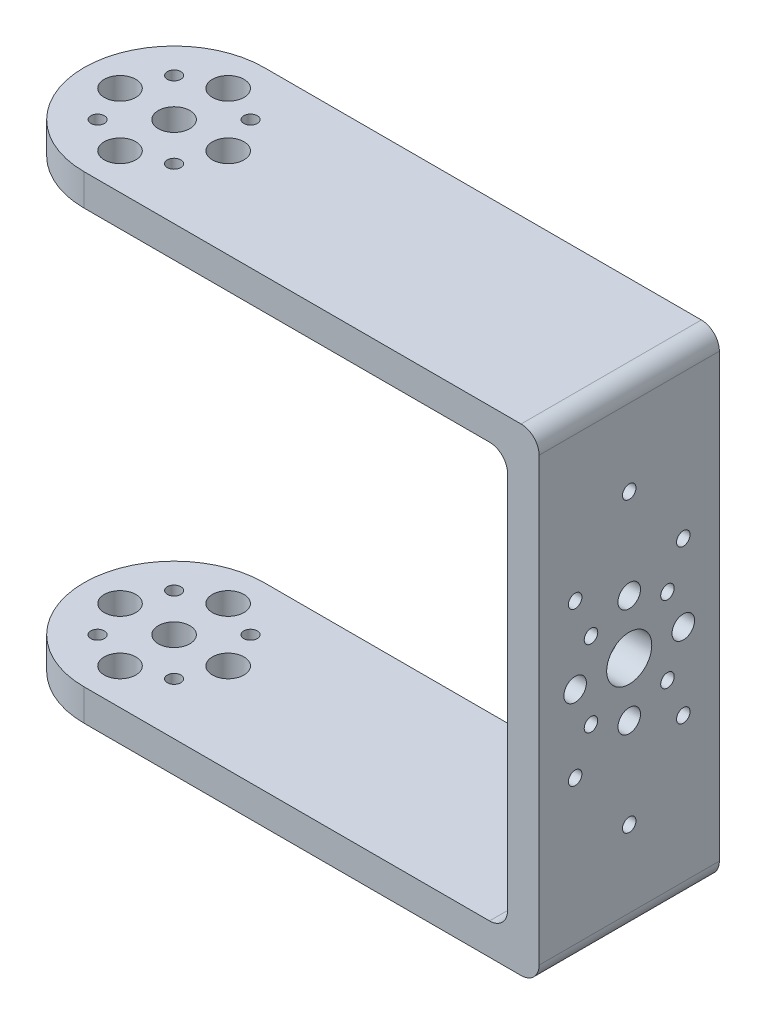
from build123d import *

# Parameters (mm, degrees)
BOSS_EXTRUDE1_DEPTH = 20
CUT_EXTRUDE1_DEPTH  = 87.499082058
SKETCH5_R           = 1.75
SKETCH5_R_2         = 0.75
CUT_EXTRUDE2_DEPTH  = 87.499082058
FILLET1_R           = 2
SKETCH6_R           = 2.5
SKETCH6_R_2         = 1.25
SKETCH6_R_3         = 0.75
CUT_EXTRUDE3_DEPTH  = 20
SKETCH7_R           = 0.75
CUT_EXTRUDE4_DEPTH  = 20
SKETCH8_R           = 0.75
CUT_EXTRUDE5_DEPTH  = 20
FILLET2_R           = 2


with BuildPart() as part:
    # Sketch2 → Boss-Extrude1 (new body)
    with BuildSketch(Plane.XY):
        Polygon((4.868885541, 24.845866319), (4.868885541, 28.345866319), (65.368885541, 28.345866319), (65.368885541, -24.654133681), (4.868885541, -24.654133681), (4.868885541, -21.154133681), (61.868885541, -21.154133681), (61.868885541, 24.845866319), align=None)
    extrude(amount=-BOSS_EXTRUDE1_DEPTH)

    # Sketch3 → Cut-Extrude1 (cut, through all)
    with BuildSketch(Plane(origin=(0, 28.345866319, 0), x_dir=(1, 0, 0), z_dir=(0, 1, 0))):
        with BuildLine():
            ThreePointArc((14.868885541, 0), (7.79781773, 2.928932188), (4.868885541, 10))
            Line((4.868885541, 10), (4.868885541, 0))
            Line((4.868885541, 0), (14.868885541, 0))
        make_face()
        with BuildLine():
            ThreePointArc((4.868885541, 10), (7.79781773, 17.071067812), (14.868885541, 20))
            Line((14.868885541, 20), (4.868885541, 20))
            Line((4.868885541, 20), (4.868885541, 10))
        make_face()
    extrude(amount=-CUT_EXTRUDE1_DEPTH, mode=Mode.SUBTRACT)

    # Sketch5 → Cut-Extrude2 (cut, through all)
    with BuildSketch(Plane(origin=(0, 28.345866319, 0), x_dir=(1, 0, 0), z_dir=(0, 1, 0))):
        with Locations(Location((14.868885541, 10, 0), (0, 0, 270))):
            Circle(SKETCH5_R)
        with Locations(Location((20.868885541, 10, 0), (0, 0, 270))):
            Circle(SKETCH5_R)
        with Locations(Location((14.868885541, 4, 0), (0, 0, 270))):
            Circle(SKETCH5_R)
        with Locations(Location((8.868885541, 10, 0), (0, 0, 270))):
            Circle(SKETCH5_R)
        with Locations(Location((14.868885541, 16, 0), (0, 0, 270))):
            Circle(SKETCH5_R)
        with Locations(Location((19.111526229, 5.757359313, 0), (0, 0, 270))):
            Circle(SKETCH5_R_2)
        with Locations(Location((10.626244854, 5.757359313, 0), (0, 0, 270))):
            Circle(SKETCH5_R_2)
        with Locations(Location((10.626244854, 14.242640687, 0), (0, 0, 270))):
            Circle(SKETCH5_R_2)
        with Locations(Location((19.111526229, 14.242640687, 0), (0, 0, 270))):
            Circle(SKETCH5_R_2)
    extrude(amount=-CUT_EXTRUDE2_DEPTH, mode=Mode.SUBTRACT)

    # Fillet1
    fillet1_edges = [part.edges().sort_by_distance(p)[0] for p in [
        (65.368885541, 28.345866319, -10),
        (65.368885541, -24.654133681, -10),
    ]]
    fillet(fillet1_edges, radius=FILLET1_R)

    # Sketch6 → Cut-Extrude3 (cut)
    with BuildSketch(Plane(origin=(65.368885541, 0, 0), x_dir=(0, 0, -1), z_dir=(1, 0, 0))):
        with Locations((10, 1.845866319)):
            Circle(SKETCH6_R)
        with Locations((10, 7.845866319)):
            Circle(SKETCH6_R_2)
        with Locations((16, 1.845866319)):
            Circle(SKETCH6_R_2)
        with Locations((10, -4.154133681)):
            Circle(SKETCH6_R_2)
        with Locations((4, 1.845866319)):
            Circle(SKETCH6_R_2)
        with Locations((14.242640687, 6.088507006)):
            Circle(SKETCH6_R_3)
        with Locations((14.242640687, -2.396774369)):
            Circle(SKETCH6_R_3)
        with Locations((5.757359313, -2.396774369)):
            Circle(SKETCH6_R_3)
        with Locations((5.757359313, 6.088507006)):
            Circle(SKETCH6_R_3)
    extrude(amount=-CUT_EXTRUDE3_DEPTH, mode=Mode.SUBTRACT)

    # Sketch7 → Cut-Extrude4 (cut)
    with BuildSketch(Plane(origin=(65.368885541, 0, 0), x_dir=(0, 0, -1), z_dir=(1, 0, 0))):
        with Locations((16, 10.345866319)):
            Circle(SKETCH7_R)
        with Locations((4, 10.345866319)):
            Circle(SKETCH7_R)
        with Locations((4, -6.654133681)):
            Circle(SKETCH7_R)
        with Locations((16, -6.654133681)):
            Circle(SKETCH7_R)
    extrude(amount=-CUT_EXTRUDE4_DEPTH, mode=Mode.SUBTRACT)

    # Sketch8 → Cut-Extrude5 (cut)
    with BuildSketch(Plane(origin=(65.368885541, 0, 0), x_dir=(0, 0, -1), z_dir=(1, 0, 0))):
        with Locations((10, 17.845866319)):
            Circle(SKETCH8_R)
        with Locations((10, -14.154133681)):
            Circle(SKETCH8_R)
    extrude(amount=-CUT_EXTRUDE5_DEPTH, mode=Mode.SUBTRACT)

    # Fillet2
    fillet2_edges = [part.edges().sort_by_distance(p)[0] for p in [
        (61.868885541, -21.154133681, -10),
        (61.868885541, 24.845866319, -10),
    ]]
    fillet(fillet2_edges, radius=FILLET2_R)


solid = part.part
